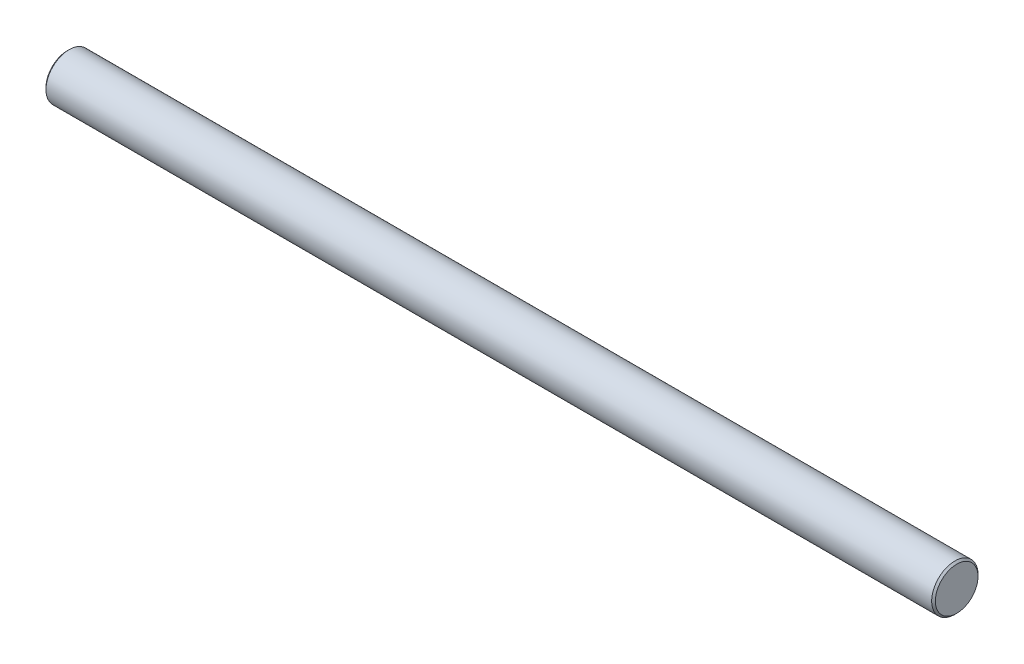
from build123d import *

# Parameters (mm, degrees)
SKETCH1_R           = 12.5
BOSS_EXTRUDE1_DEPTH = 480
CHAMFER1_SIZE       = 1


with BuildPart() as part:
    # Sketch1 → Boss-Extrude1 (new body)
    with BuildSketch(Plane(origin=(0, 0, 0), x_dir=(0, 0, -1), z_dir=(1, 0, 0))):
        Circle(SKETCH1_R)
    extrude(amount=BOSS_EXTRUDE1_DEPTH)

    # Chamfer1
    chamfer1_edges = [part.edges().sort_by_distance(p)[0] for p in [
        (0, 0, 12.5),
        (480, 0, 12.5),
    ]]
    chamfer(chamfer1_edges, length=CHAMFER1_SIZE)


solid = part.part
